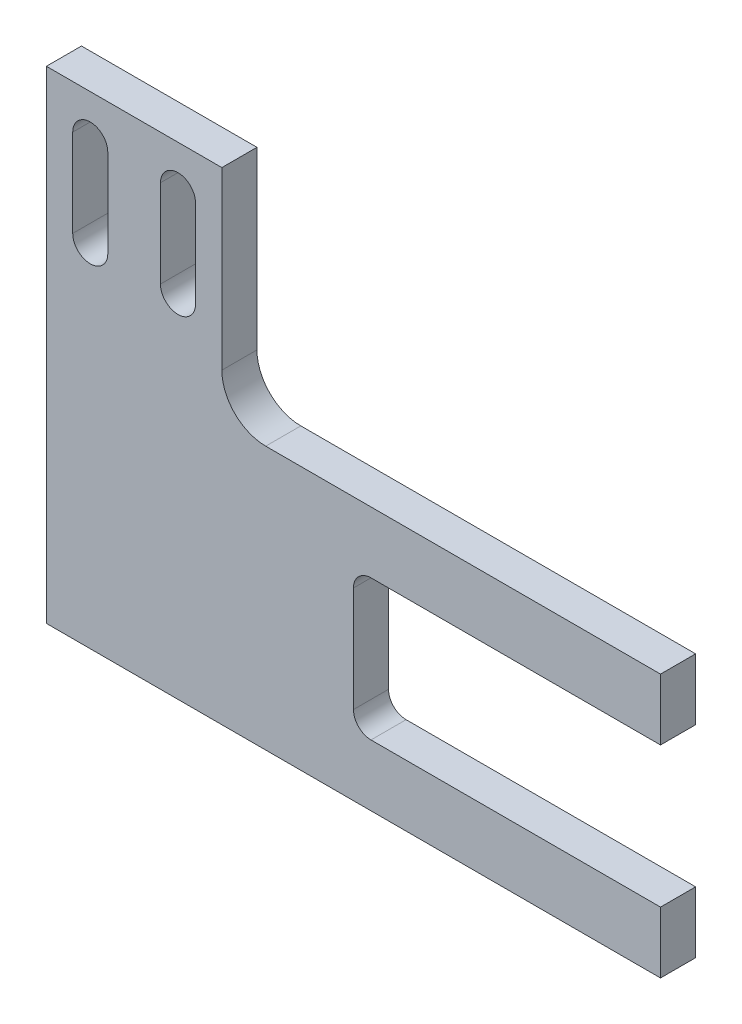
from build123d import *

# Parameters (mm, degrees)
EXTRUDE_1_DEPTH     = 4
CUT_EXTRUDE_1_REACH = 91.112
FILLET_1_R          = 5
CUT_EXTRUDE_2_REACH = 91.112
SKETCH_3_W          = 35
SKETCH_3_H          = 16
FILLET_2_R          = 2


with BuildPart() as part:
    # 草图1 → 凸台-拉伸1 (new body)
    with BuildSketch(Plane.XY):
        Polygon((0, 0), (0, -55), (70, -55), (70, -25), (20, -25), (20, 0), align=None)
    extrude(amount=EXTRUDE_1_DEPTH)

    # 草图2 → 切除-拉伸1 (cut, up to next)
    with BuildSketch(Plane.XY.offset(4), mode=Mode.PRIVATE) as cut_extrude_1_sk1:
        with BuildLine():
            Line((3, -15), (3, -5))
            ThreePointArc((3, -5), (5, -3), (7, -5))
            Line((7, -5), (7, -15))
            ThreePointArc((7, -15), (5, -17), (3, -15))
        make_face()
    cut_extrude_1_tool1 = extrude(cut_extrude_1_sk1.sketch, amount=-CUT_EXTRUDE_1_REACH, mode=Mode.PRIVATE) & part.part
    # 草图2 → 切除-拉伸1 (cut, up to next)
    with BuildSketch(Plane.XY.offset(4), mode=Mode.PRIVATE) as cut_extrude_1_sk2:
        with BuildLine():
            Line((13, -15), (13, -5))
            ThreePointArc((13, -5), (15, -3), (17, -5))
            Line((17, -5), (17, -15))
            ThreePointArc((17, -15), (15, -17), (13, -15))
        make_face()
    cut_extrude_1_tool2 = extrude(cut_extrude_1_sk2.sketch, amount=-CUT_EXTRUDE_1_REACH, mode=Mode.PRIVATE) & part.part
    add(cut_extrude_1_tool1.solids().sort_by_distance((5, -10, 4))[0], mode=Mode.SUBTRACT)
    add(cut_extrude_1_tool2.solids().sort_by_distance((15, -10, 4))[0], mode=Mode.SUBTRACT)

    # 圆角1
    fillet_1_edges = [part.edges().sort_by_distance(p)[0] for p in [
        (20, -25, 2),
    ]]
    fillet(fillet_1_edges, radius=FILLET_1_R)

    # 草图3 → 切除-拉伸2 (cut, up to next)
    with BuildSketch(Plane.XY.offset(4), mode=Mode.PRIVATE) as cut_extrude_2_sk1:
        with Locations((52.5, -40)):
            Rectangle(SKETCH_3_W, SKETCH_3_H)
    cut_extrude_2_tool1 = extrude(cut_extrude_2_sk1.sketch, amount=-CUT_EXTRUDE_2_REACH, mode=Mode.PRIVATE) & part.part
    add(cut_extrude_2_tool1.solids().sort_by_distance((52.5, -40, 4))[0], mode=Mode.SUBTRACT)

    # 圆角2
    fillet_2_edges = [part.edges().sort_by_distance(p)[0] for p in [
        (35, -48, 2),
        (35, -32, 2),
    ]]
    fillet(fillet_2_edges, radius=FILLET_2_R)


solid = part.part
